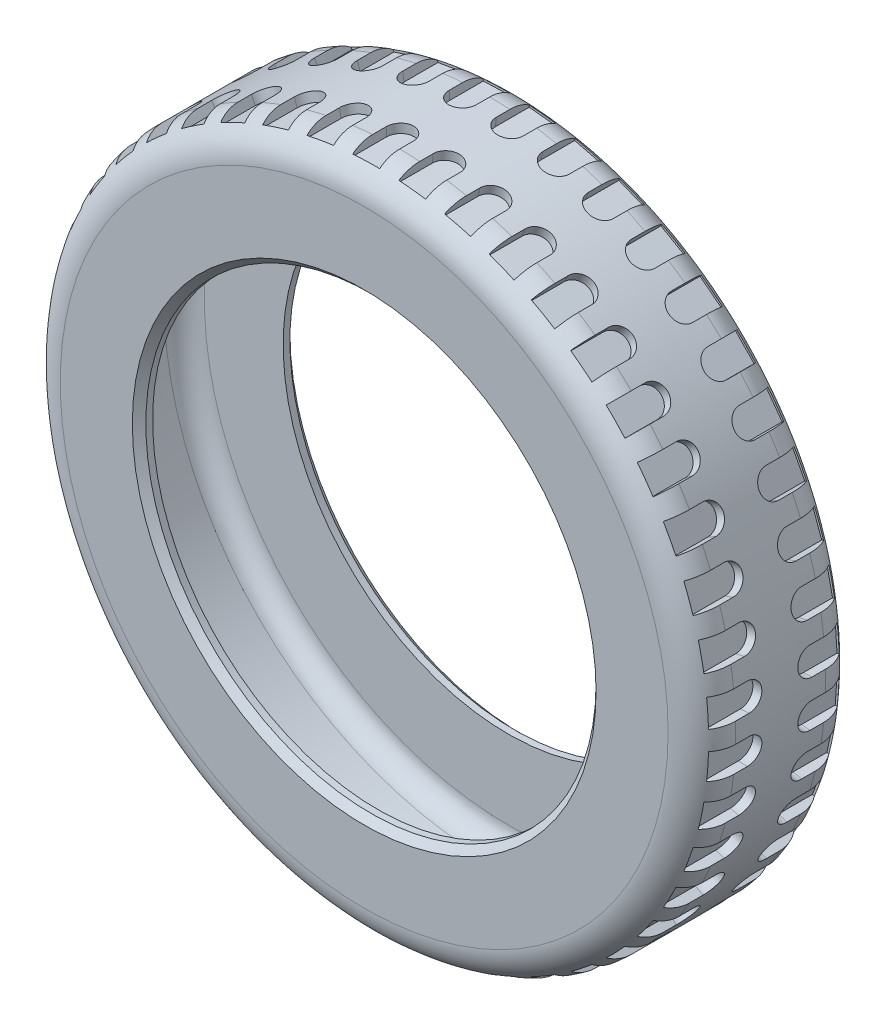
from build123d import *

# Parameters (mm, degrees)
SKETCH1_R           = 7.5
SKETCH1_R_2         = 5
BOSS_EXTRUDE1_DEPTH = 1.75
FILLET1_R           = 0.75
SHELL1_T            = -0.3
CHAMFER1_SIZE       = 0.15
CUT_EXTRUDE1_START  = -15.3
CUT_EXTRUDE1_DEPTH  = 8
CIRPATTERN1_COUNT   = 45


with BuildPart() as part:
    # Sketch1 → Boss-Extrude1 (new, symmetric)
    with BuildSketch(Plane.XY):
        Circle(SKETCH1_R)
        Circle(SKETCH1_R_2, mode=Mode.SUBTRACT)
    extrude(amount=BOSS_EXTRUDE1_DEPTH, both=True)

    # Fillet1
    fillet1_edges = [part.edges().sort_by_distance(p)[0] for p in [
        (-7.5, 0, -1.75),
        (-7.5, 0, 1.75),
    ]]
    fillet(fillet1_edges, radius=FILLET1_R)

    # Shell1
    shell1_openings = [part.faces().sort_by_distance(p)[0] for p in [
        (-5, 0, 0),
    ]]
    offset(amount=SHELL1_T, openings=shell1_openings, kind=Kind.INTERSECTION)

    # Chamfer1
    chamfer1_edges = [part.edges().sort_by_distance(p)[0] for p in [
        (-5, 0, -1.75),
        (-5, 0, 1.75),
    ]]
    chamfer(chamfer1_edges, length=CHAMFER1_SIZE)

    # Sketch2 → Cut-Extrude1 (cut)
    with BuildSketch(Plane(origin=(0, 0, 0), x_dir=(0, 0, -1), z_dir=(1, 0, 0)).offset(CUT_EXTRUDE1_START)):
        with BuildLine():
            Line((-0.7, 0.3), (-1.45, 0.3))
            Line((-1.45, 0.3), (-1.45, -0.3))
            Line((-1.45, -0.3), (-0.7, -0.3))
            ThreePointArc((-0.7, -0.3), (-0.4, 0), (-0.7, 0.3))
        make_face()
        with BuildLine():
            Line((1.45, -0.3), (0.7, -0.3))
            ThreePointArc((0.7, -0.3), (0.4, 0), (0.7, 0.3))
            Line((0.7, 0.3), (1.45, 0.3))
            Line((1.45, 0.3), (1.45, -0.3))
        make_face()
    cut_extrude1 = extrude(amount=CUT_EXTRUDE1_DEPTH, mode=Mode.SUBTRACT)

    # CirPattern1: Cut-Extrude1 ×45 about axis
    cirpattern1_axis = Axis((0, 0, 0), (0, 0, 1))
    for i in range(1, CIRPATTERN1_COUNT):
        add(cut_extrude1.rotate(cirpattern1_axis, i * 360 / CIRPATTERN1_COUNT), mode=Mode.SUBTRACT)


solid = part.part
